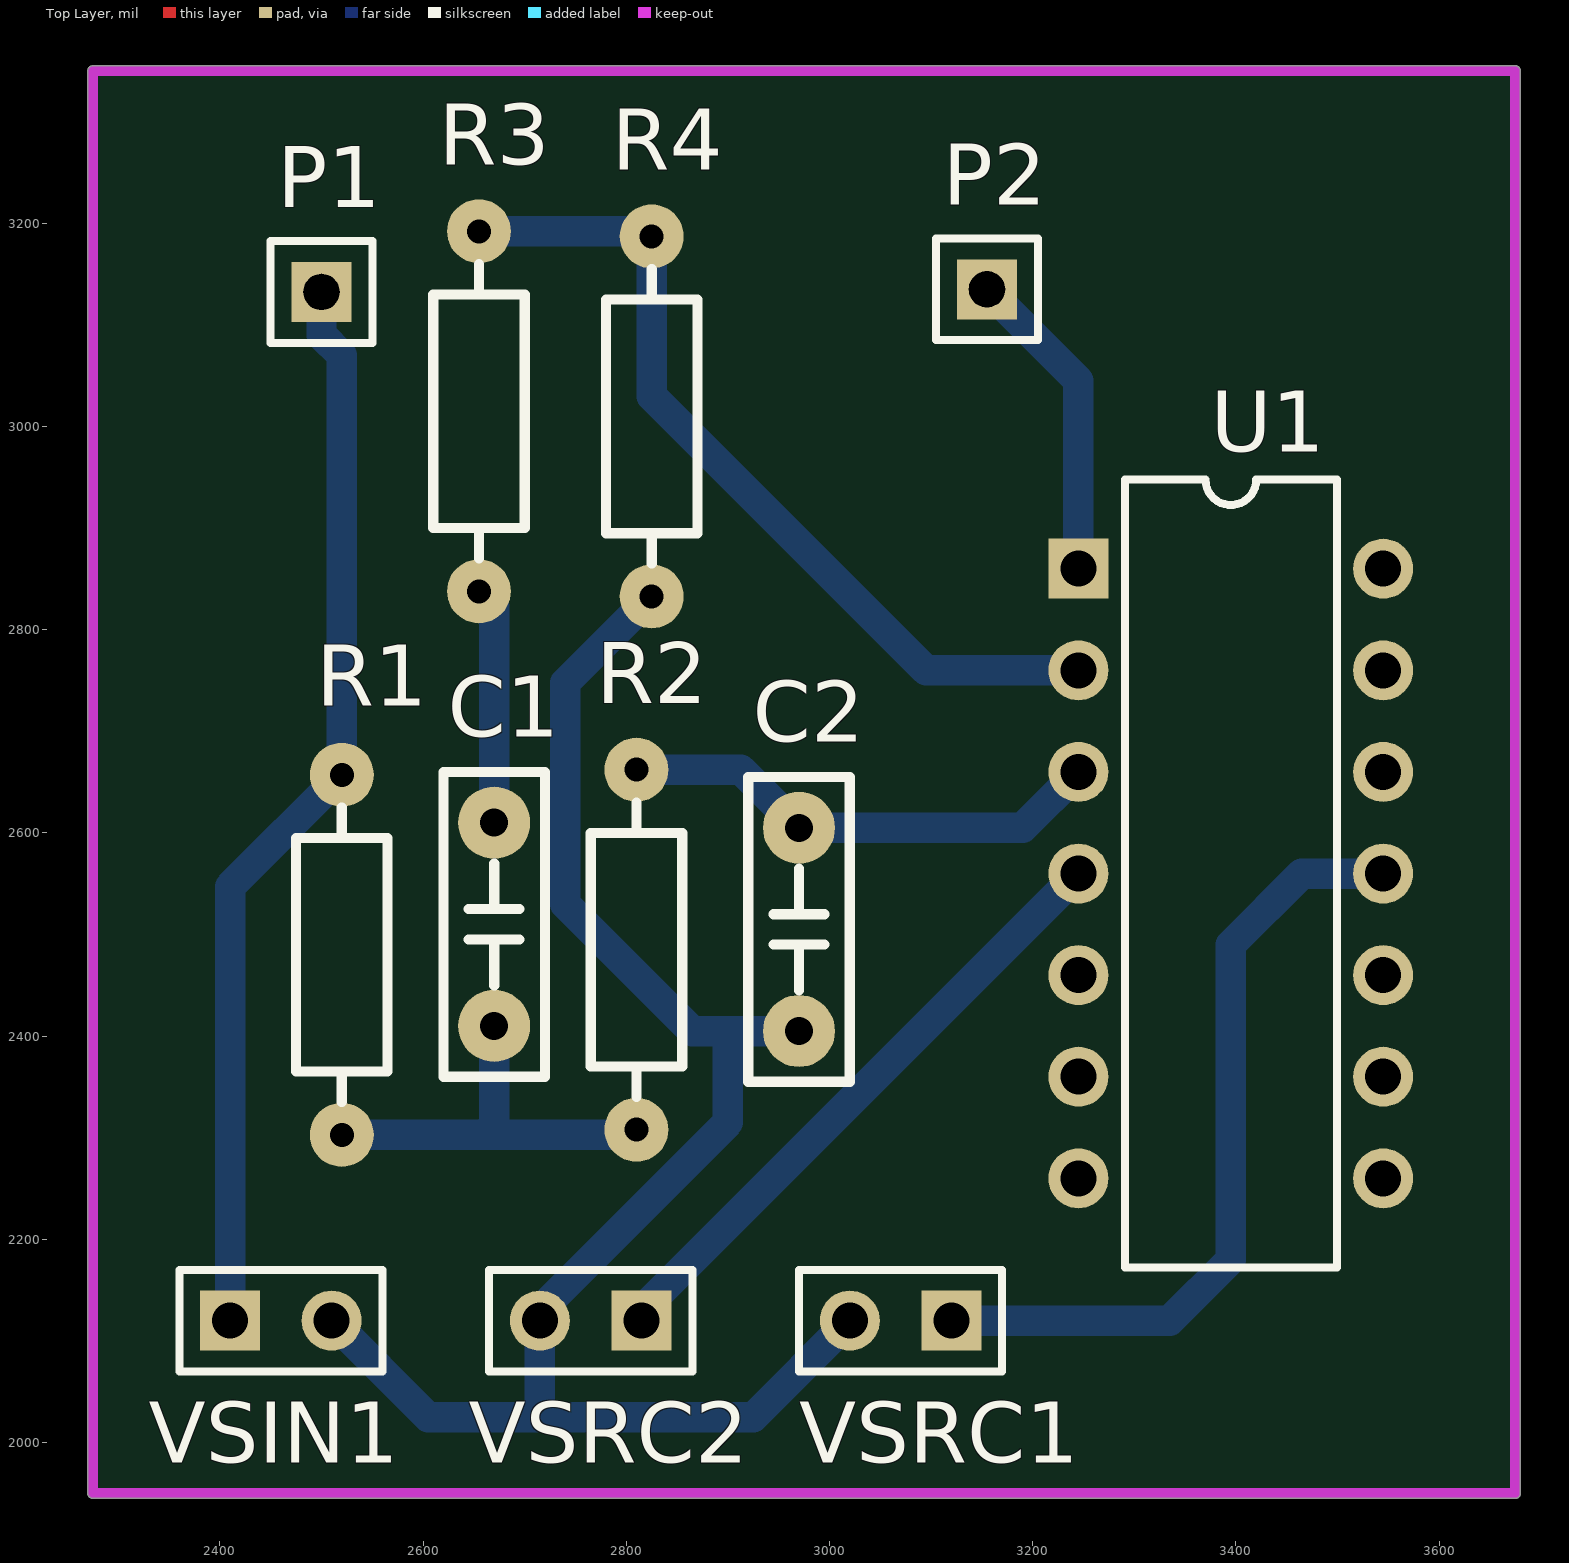
[diagram p0: Top Layer view]
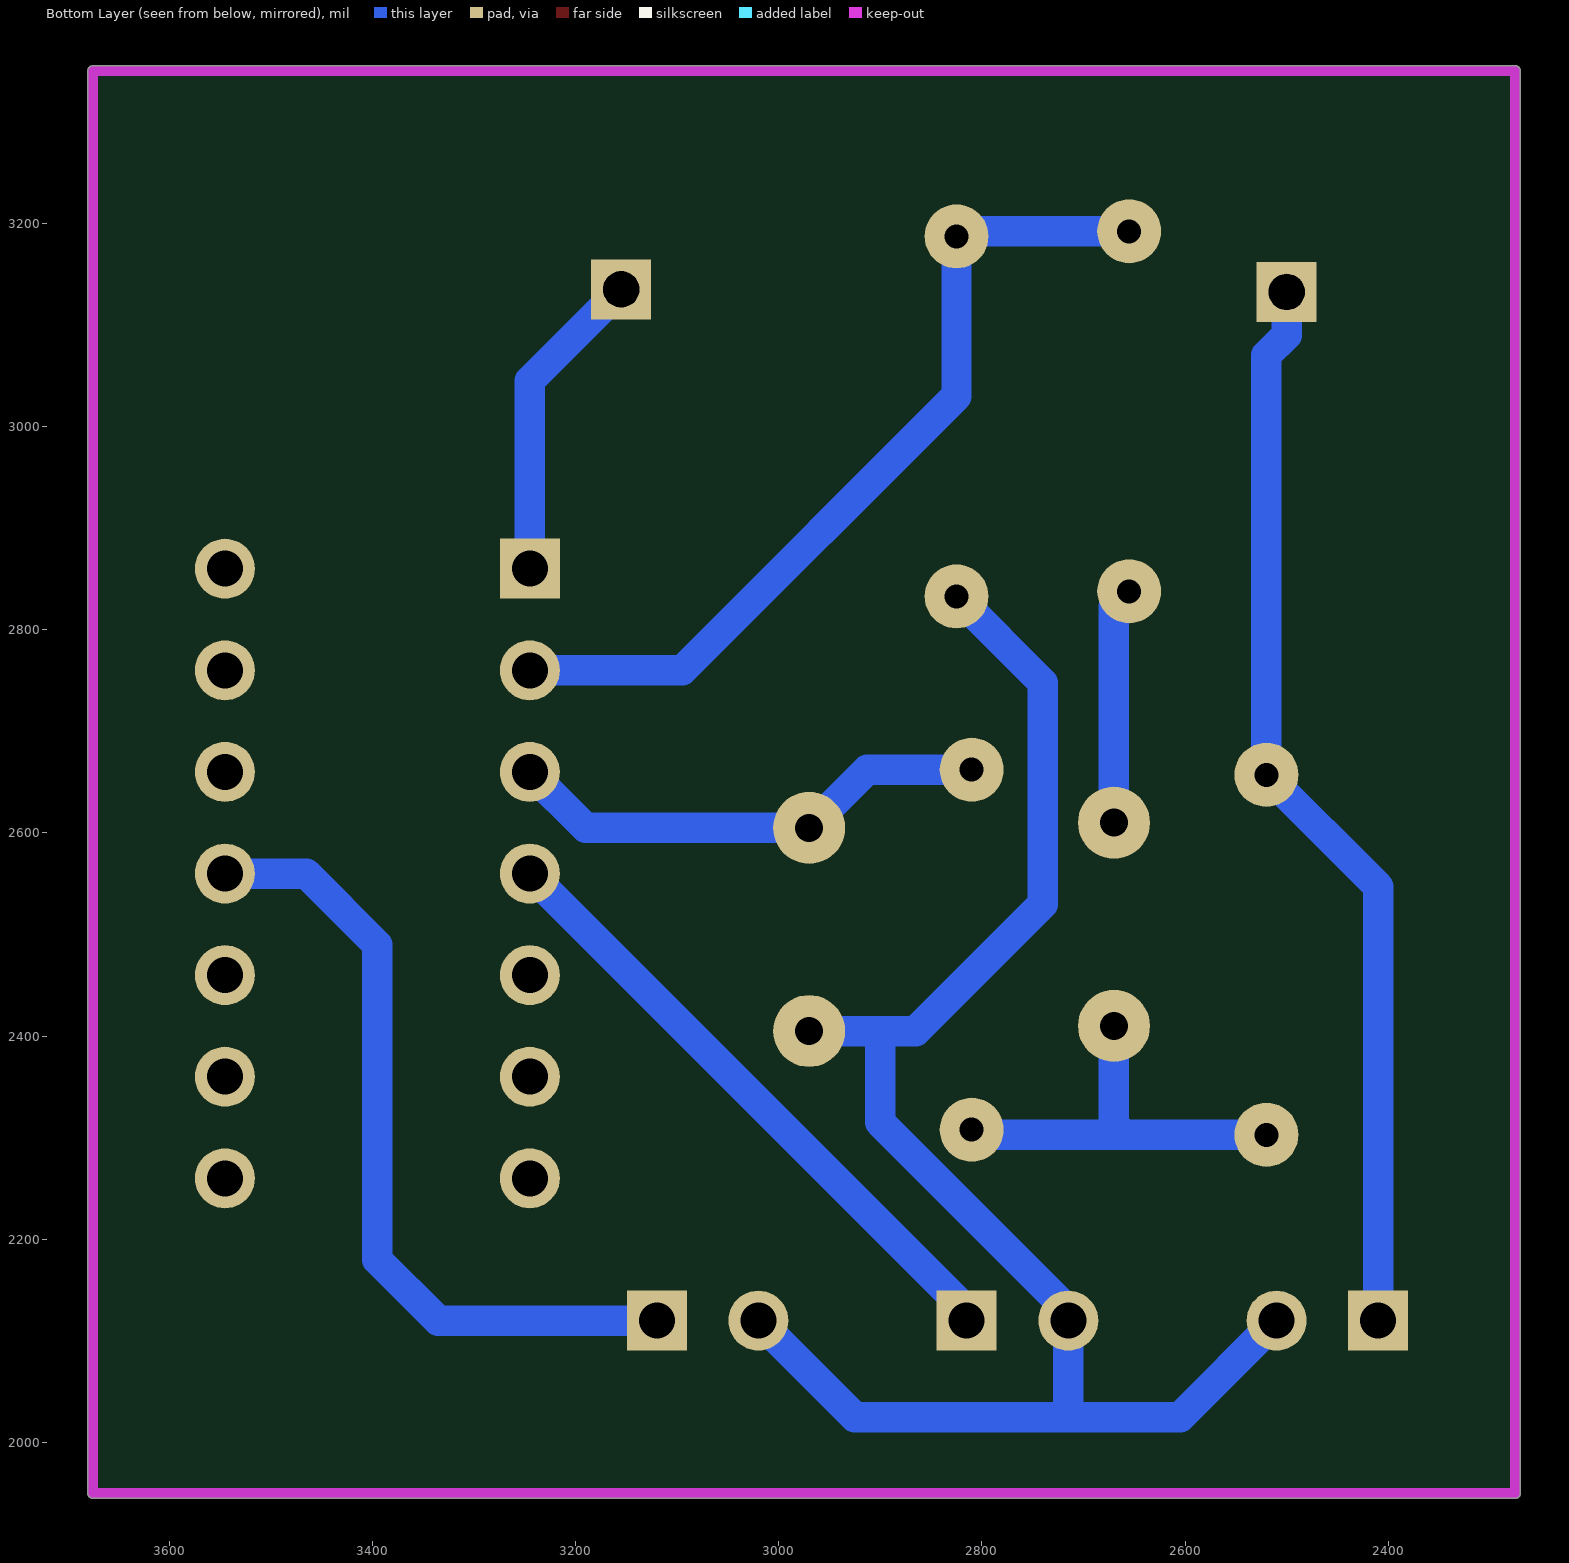
[diagram p1: Bottom Layer view, seen from below]
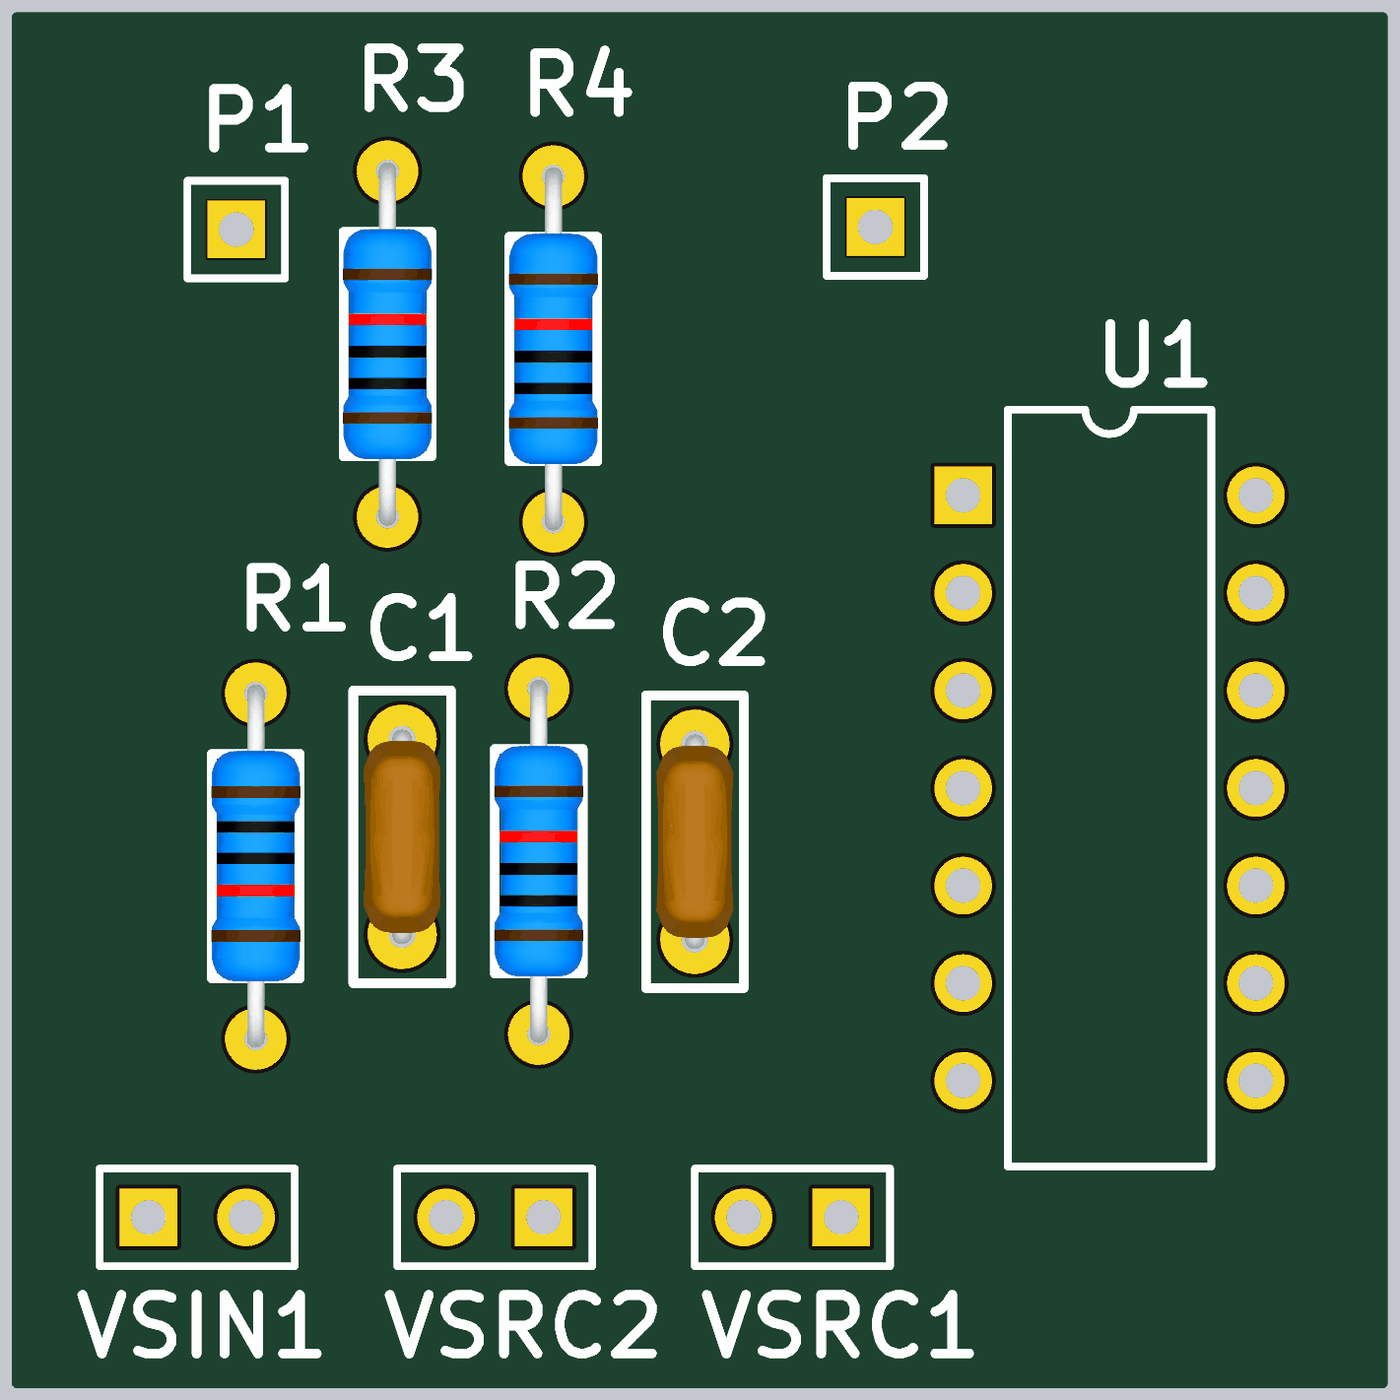
[diagram p2: 3D render of the assembled board from above, using the file's embedded part models]
# Altium PCB MISC80827.PcbDoc
Units mil, origin at the board's own origin, x right, y up, seen from the top; angles counter-clockwise.
Board outline 1410.03 x 1410.03 mil, 2 copper layers (Top Layer, Bottom Layer); 12 components, 9 nets, 34 pads, 0 vias.

## Layer stack, top to bottom (the 12.6 mil dielectric is the usual default, probably not edited)
Top Solder: solder mask 0.4, Solder Resist, Dk 3.5
Top Layer: signal copper 1.4
Dielectric 1: dielectric 12.6, FR-4, Dk 4.8
Bottom Layer: signal copper 1.4
Bottom Solder: solder mask 0.4, Solder Resist, Dk 3.5

## Board outline
2269.99,1950 ccw(c2275,1950) 2275,1944.98 3675,1944.98 ccw(c3675,1950) 3680.01,1950 3680.01,3350 ccw(c3675,3350) 3675,3355.01 2275,3355.01 ccw(c2275,3350) 2269.99,3350

## Design rules (kind name [scope] priority, off if disabled: settings)
Clearance [All] p1: gap=10
MinimumSolderMaskSliver [All] p1: minsoldermaskwidth=0
PolygonConnect [All] p1: connectstyle=Relief reliefconductorwidth=10 reliefentries=4 polygonreliefangle="90 Angle" airgapwidth=10
RoutingVias [All] p1: holewidth=28 width=50 viastyle="Through Hole" minholewidth=28 minwidth=50 maxholewidth=28 maxwidth=50
SilkToSilkClearance [All] p1: silktosilkclearance=0
SilkToSolderMaskClearance [IsPad] p1: minsilkscreentomaskgap=0 clearancetoexposedcopper=TRUE
SolderMaskExpansion [All] p1: expansion=4
Width [All] p1: maxlimit=30 minlimit=10 preferedwidth=10
27 further rules are at their usual default settings.

## Components (designator, comment, footprint, x,y, rotation, side; value= is the part's Value field where it differs from the comment)
C1 "0.1UF" MLCC5.08-A 2670,2510 r90 top
C2 "0.1UF" MLCC5.08-A 2970,2505 r90 top
P1 "HDR1X1" HDR1X1 2500,3132.41 r0 top
P2 "HDR1X1" HDR1X1 3155,3135 r0 top
R1 "796" "RS 1/4W" 2520,2480 r270 top
R2 "796" "RS 1/4W" 2810,2485 r90 top
R3 "3.184K" "RS 1/4W" 2655,3015 r90 top
R4 "3.184K" "RS 1/4W" 2825,3010 r90 top
U1 "LM324N" 646-06 3395,2560 r270 top
VSIN1 "1000HZ" HDR1X2 2410,2120 r0 top
VSRC1 "12Vneg" HDR1X2 3120,2120 r180 top
VSRC2 "12Vpos" HDR1X2 2815,2120 r180 top

## Footprints (in the part's own frame and the unit in brackets; to place one, negate y for a bottom-side part, rotate by r counter-clockwise, add the part's x,y. Pads: shape width x height; smd on the part's side, far side on the other; paste and mask are expansions set on the pad)
646-06 [mm] "DIP; 14 Leads; Row Spacing 7.62 mm; Pitch 2.54 mm"
  rect 1.5x1.5 hole 0.9: 1(-7.62,-3.81)
  round 1.5 hole 0.9: 2(-5.08,-3.81) 3(-2.54,-3.81) 4(0,-3.81) 5(2.54,-3.81) 6(5.08,-3.81) 7(7.62,-3.81) 8(7.62,3.81) 9(5.08,3.81) 10(2.54,3.81) 11(0,3.81) 12(-2.54,3.81) 13(-5.08,3.81) 14(-7.62,3.81)
  silkscreen extent -9.85,-2.65 9.85,2.65
HDR1X1 [mm]
  rect 1.5x1.5 hole 0.9 slot 0.905 at 0 deg paste+0 mask+0.051: 1(0,0)
  silkscreen extent -1.27,-1.27 1.27,1.27
HDR1X2 [mm] "Connector; Header; 2 Position"
  rect 1.5x1.5 hole 0.9: 1(0,0)
  round 1.5 hole 0.9: 2(2.54,0)
  silkscreen extent -1.27,-1.27 3.81,1.27
MLCC5.08-A [mm] "独石电容，脚距5.08mm"
  round 1.8 hole 0.7: 1(-2.54,0) 2(2.54,0)
  silkscreen extent -3.81,-1.27 3.81,1.27, body extent -2.79,-1 2.79,1, height 3.71
"RS 1/4W" [mm] "直插色环电阻，脚距9mm，直径2.3mm"
  round 1.6 hole 0.6: 1(-4.5,0) 2(4.5,0)
  silkscreen extent -3.68,-1.14 3.68,1.14, body extent -4.72,-1.16 4.73,1.16, height 2.32

## Part data
C1 C2: library part C-MLCC, "Monolithic ceramic capacitor"
R1 R2 R3 R4: library part R-S, "Color-band resistor"
U1: "Quad Low-Power Operational Amplifier"
VSIN1 VSRC1 VSRC2: library part 电流源

## Nets (pads, with @x,y where several pads share a name; then routed paths per layer and width w, separated by ;. In a path a pad name is that pad's centre, name@x,y a point inside that pad or via, vN(x,y) a via of type N, cw(c..) or ccw(c..) an arc to the next point about the centre after c; other vN are vias at no path point)
GND: C2.1 R4.1 VSIN1.2 VSRC1.2 VSRC2.2 | length 1667.2
  Bottom Layer w30: VSIN1.2 2605,2025 2710,2025 ; R4.1 2740,2747.83 2740,2530 2865,2405 2900,2405 ; C2.1 2900,2405 ; VSRC1.2 2925,2025 2710,2025 ; 2710,2025 2715,2030 VSRC2.2 2715,2130 2900,2315 2900,2405
INPUT: P1.1 R1.1 VSIN1.1 | length 1066.3
  Bottom Layer w30: VSIN1.1 2410,2547.17 R1.1 2520,3070 2500,3090 P1.1
NetC1_1: C1.1 R1.2 R2.1 | length 403.4
  Bottom Layer w30: R1.2 2660,2302.83 ; C1.1 2670,2312.83 2660,2302.83 ; R2.1 2805,2302.83 2660,2302.83
NetC1_2: C1.2 R3.1 | length 234
  Bottom Layer w30: R3.1 2670,2822.83 C1.2
NetC2_2: C2.2 R2.2 U1.3 | length 481.5
  Bottom Layer w30: R2.2 2912.83,2662.17 C2.2 3190,2605 U1.3
NetR3_2: R3.2 R4.2 U1.2 | length 861.1
  Bottom Layer w30: R3.2 2820,3192.17 R4.2 2825,3030 3095,2760 U1.2
NetU1_4: U1.4 VSRC2.1 | length 618.1
  Bottom Layer w30: VSRC2.1 2815,2130 U1.4
NetU1_11: U1.11 VSRC1.1 | length 788.8
  Bottom Layer w30: VSRC1.1 3335,2120 3395,2180 3395,2490 3465,2560 U1.11
OUTPUT: P2.1 U1.1 | length 312.3
  Bottom Layer w30: P2.1 3245,3045 U1.1
pads on no net: U1.5 U1.6 U1.7 U1.8 U1.9 U1.10 U1.12 U1.13 U1.14

## Keep-outs
Keep-Out Layer:
  lines w10: 2630,3350 3625,3350 3675,3350 3675,1950 2275,1950 2275,3350 2665,3350